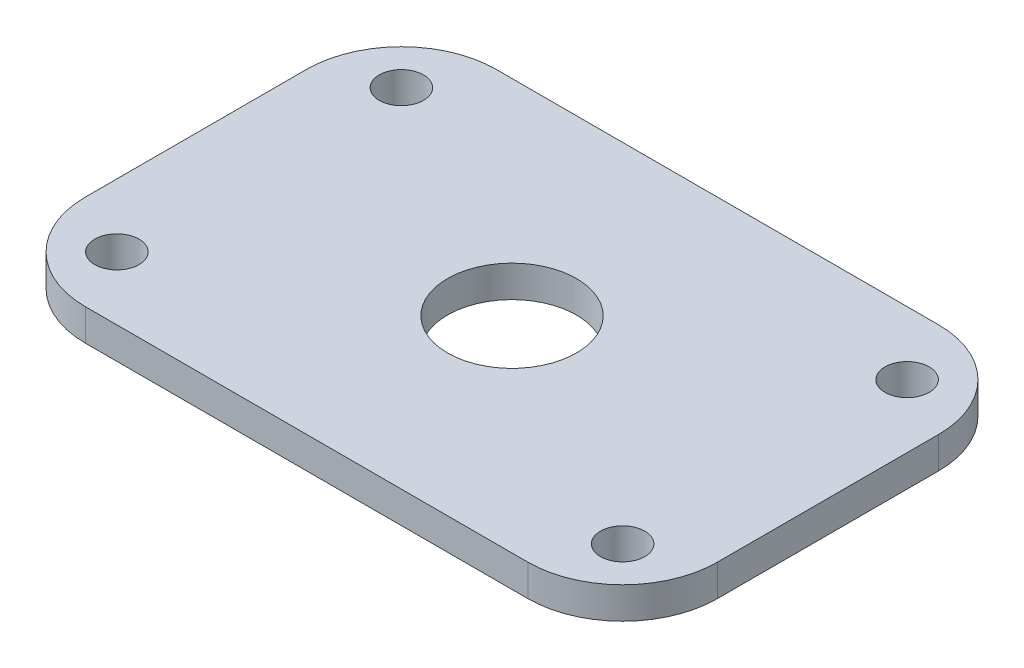
from build123d import *

# Parameters (mm, degrees)
BOSS_EXTRUDE1_DEPTH          = 5
M24_TAPPED_HOLE2_D           = 20.4
M24_TAPPED_HOLE2_ON_FACE_2_D = 20.4
HOLE1_D                      = 7
LPATTERN1_COUNT              = 2
LPATTERN1_PITCH              = 80
LPATTERN1_COUNT_DIR2         = 2
LPATTERN1_PITCH_DIR2         = 45


with BuildPart() as part:
    # Sketch1 → Boss-Extrude1 (new body)
    with BuildSketch(Plane(origin=(0, 0, 0), x_dir=(1, 0, 0), z_dir=(0, 1, 0))):
        with BuildLine():
            Line((-35, 32.5), (35, 32.5))
            ThreePointArc((35, 32.5), (45.606601718, 28.106601718), (50, 17.5))
            Line((50, 17.5), (50, -17.5))
            ThreePointArc((50, -17.5), (45.606601718, -28.106601718), (35, -32.5))
            Line((35, -32.5), (-35, -32.5))
            ThreePointArc((-35, -32.5), (-45.606601718, -28.106601718), (-50, -17.5))
            Line((-50, -17.5), (-50, 17.5))
            ThreePointArc((-50, 17.5), (-45.606601718, 28.106601718), (-35, 32.5))
        make_face()
    extrude(amount=BOSS_EXTRUDE1_DEPTH)

    # M24 Tapped Hole2 (through all)
    with Locations(Plane(origin=(0, 0, 0), x_dir=(0, 0, -1), z_dir=(0, -1, 0))):
        with Locations((0, 0)):
            Hole(M24_TAPPED_HOLE2_D / 2)

    # M24 Tapped Hole2 on face 2 (through all)
    with Locations(Plane.ZX.offset(5)):
        with Locations((0, 0)):
            Hole(M24_TAPPED_HOLE2_ON_FACE_2_D / 2)

    # Hole1 (through all)
    with Locations(Plane(origin=(-40, 5, -22.5), x_dir=(0, 0, 1), z_dir=(0, 1, 0))):
        with Locations((0, 0)):
            hole1 = Hole(HOLE1_D / 2)

    # LPattern1: Hole1 2 × 2
    with Locations(*[(i * LPATTERN1_PITCH, 0, j * LPATTERN1_PITCH_DIR2) for i in range(LPATTERN1_COUNT) for j in range(LPATTERN1_COUNT_DIR2) if (i, j) != (0, 0)]):
        add(hole1, mode=Mode.SUBTRACT)


solid = part.part
